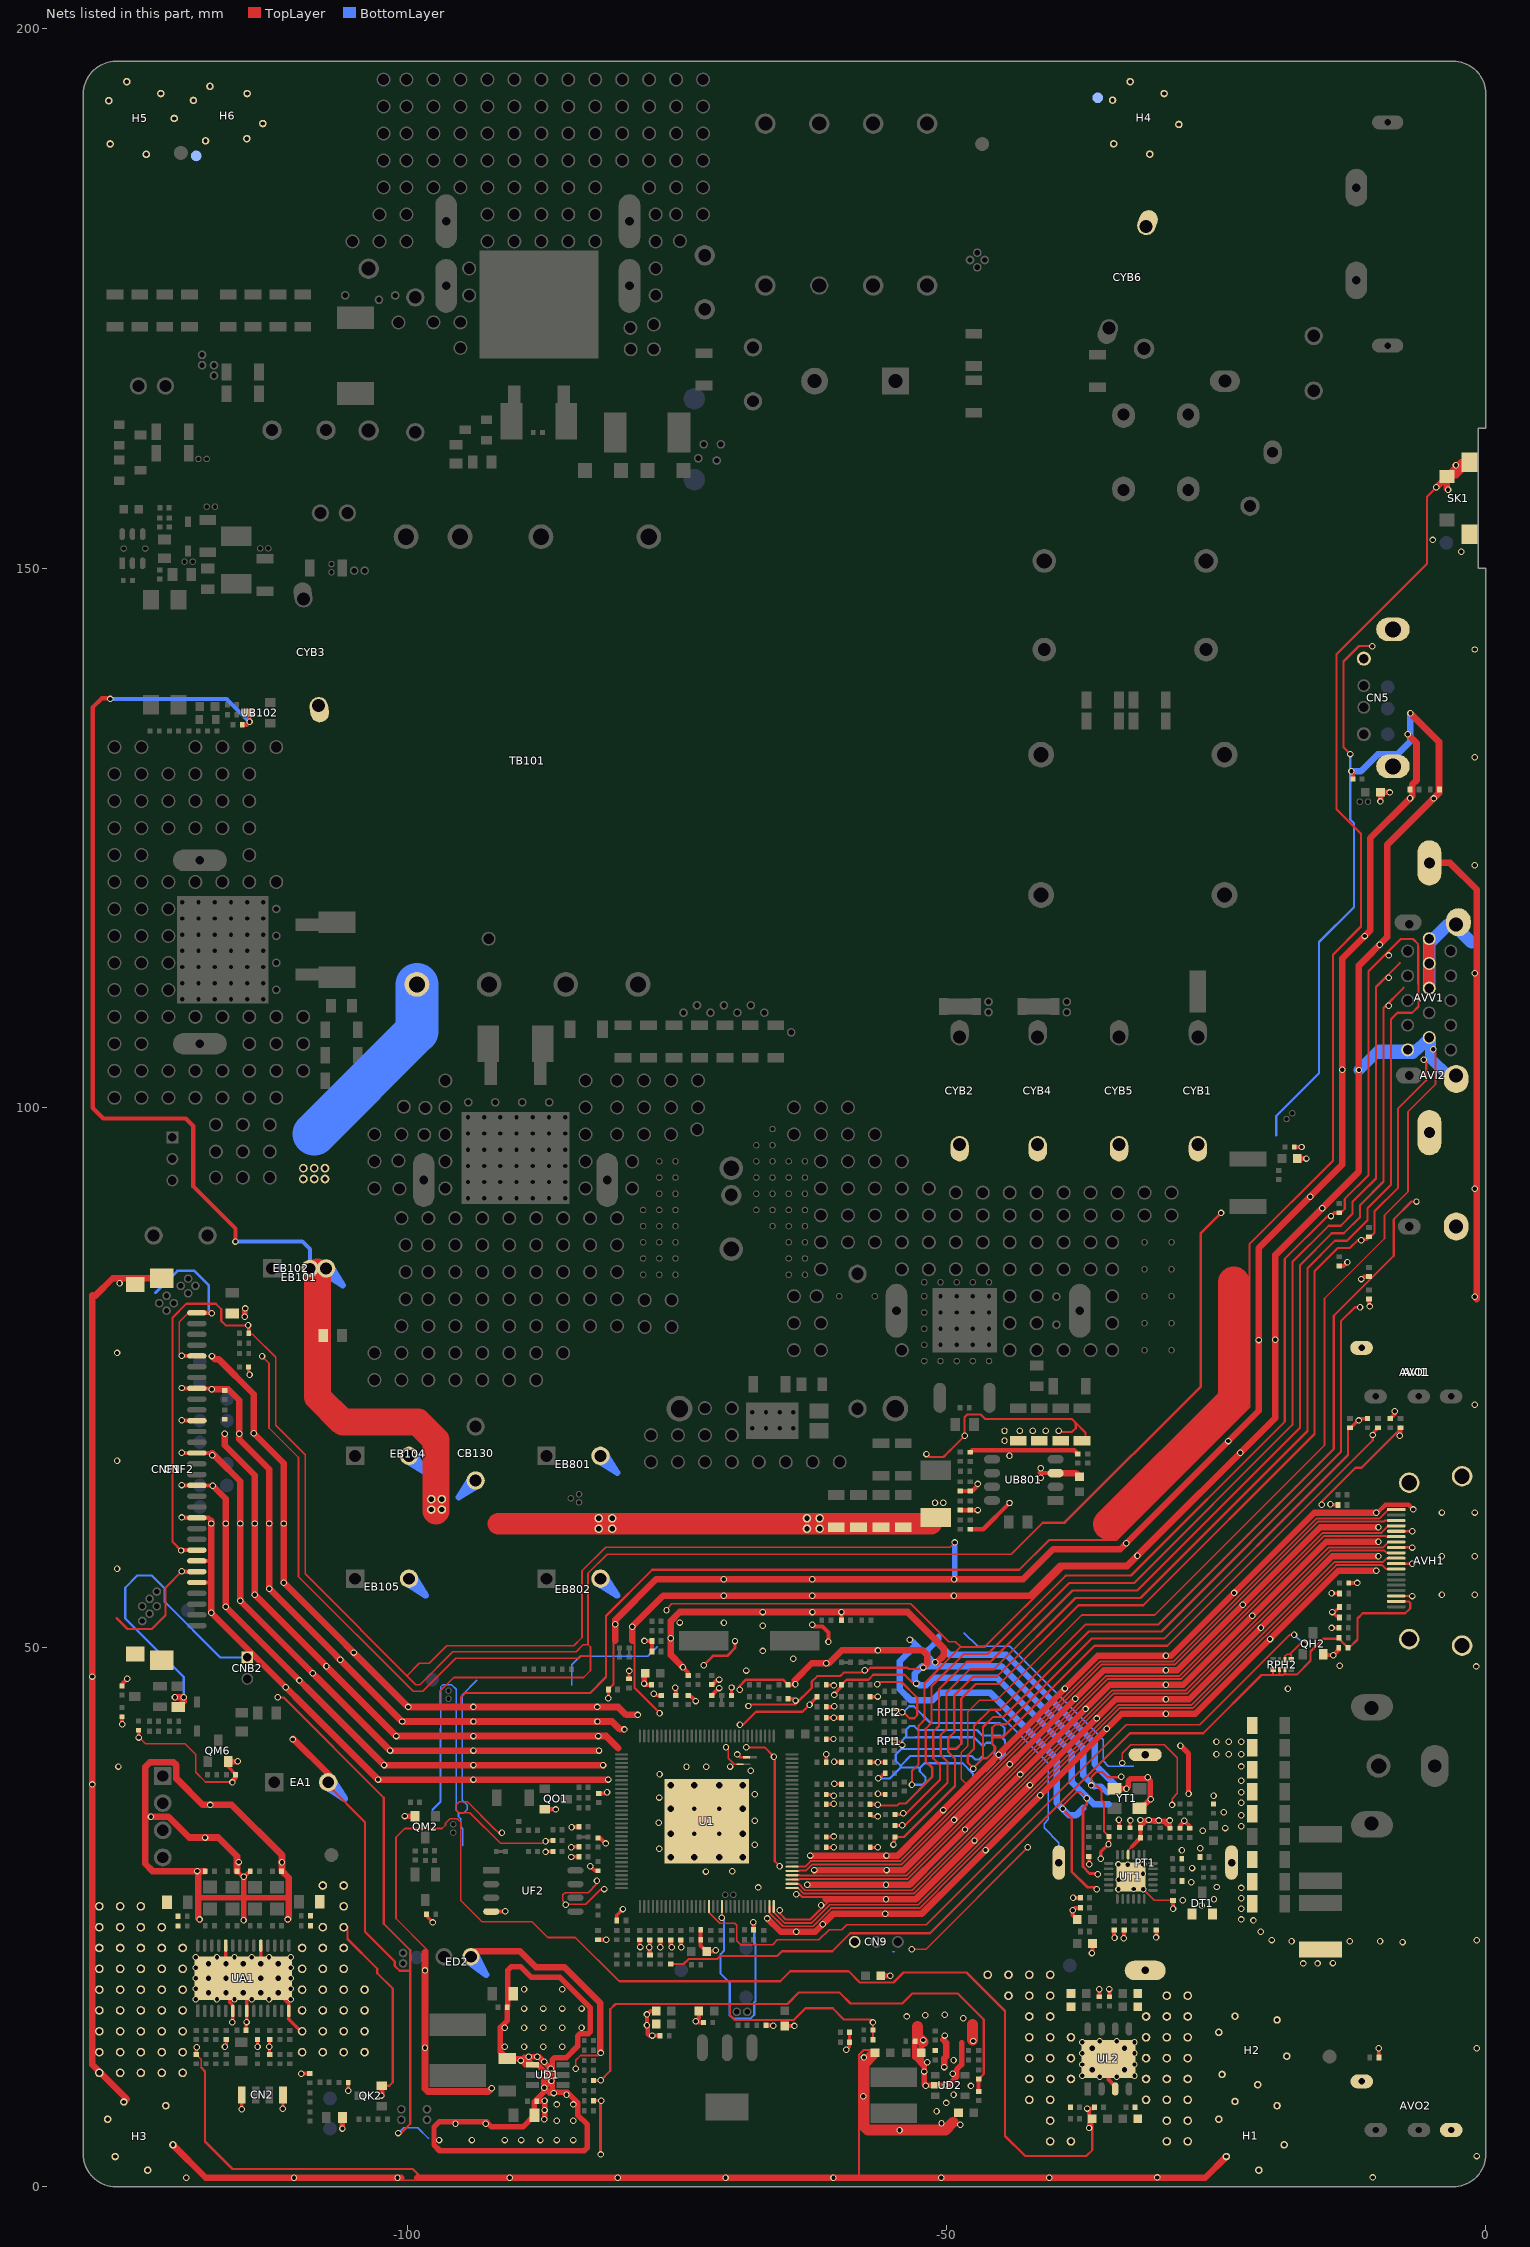
[diagram p0: the nets of this part, all layers, seen from the top]
# Altium PCB MISC84438.PcbDoc (part 10 of 15)
Units mm, origin at the board's own origin, x right, y up, seen from the top; angles counter-clockwise.
Board outline 130 x 197 mm, 2 copper layers (TopLayer, BottomLayer), stack 1.571 mm thick; 574 components, 314 nets, 2636 pads, 811 vias.

## Via types
v1: diameter 0.6, hole 0.4, TopLayer to BottomLayer, tented both sides, 780 vias
v2: diameter 0.7, hole 0.5, TopLayer to BottomLayer, tented both sides, 15 vias
v3: diameter 0.8, hole 0.6, TopLayer to BottomLayer, tented both sides, 12 vias
v4: diameter 0.8, hole 0.5, TopLayer to BottomLayer, tented both sides, 4 vias

## Nets (pads, with @x,y where several pads share a name; then routed paths per layer and width w, separated by ;. In a path a pad name is that pad's centre, name@x,y a point inside that pad or via, vN(x,y) a via of type N, cw(c..) or ccw(c..) an arc to the next point about the centre after c; other vN are vias at no path point) (continued)
GND: (continued)
  TopLayer w0.381: CF38.2@-126.416,43.555 -126.416,42.901 v1(-126.39,42.875) ; CM4.2@-126.416,46.412 -126.416,46.584 v1(-125.933,47.066) ; v1@-120.913,59 CNF2.23@-119.486,59 ; v1(-120.886,57.029) -120.857,57 CNF2.25@-119.486,57 ; v1(-120.886,62.029) -120.857,62 CNF2.20@-119.486,62 -118.413,62 v1@-118.154,61.741 ; v1(-120.886,65.029) -120.857,65 CNF2.17@-119.486,65 -118.04,65 v1(-118.001,64.96) ; v1(-120.886,68.029) -120.857,68 CNF2.14@-119.486,68 -118.31,68 -118.102,67.793 v1(-118.051,67.793) ; v1(-120.886,71.029) -120.857,71 CNF2.11@-119.486,71 ; v1(-120.886,74.029) -120.857,74 CNF2.8@-119.486,74 -118.196,74 v1(-118.11,73.914) ; v1(-120.886,77.029) -120.857,77 CNF2.5@-119.486,77 ; CNF2.26@-119.486,56 -118.115,56 ; CNF2.24@-119.486,58 -118.115,58 ; CNF2.1@-119.486,81 -118.115,81 v1@-118.086,80.971 ; v1(-116.18,37.465) -116.18,37.554 -115.882,37.852 ; CA5.2@-115.766,29.248 -115.245,28.727 v1(-115.138,28.727) -115.054,28.727 CA10.2@-114.533,29.248 ; v1(-109.791,10.477) -109.786,10.483 CK4.2@-109.004,10.483 ; UF2.4@-92.19,25.502 -90.932,25.502 v1(-90.907,25.527) ; -89.035,11.301 UD1.1@-88.356,11.301 ; QO1.E@-87.224,34.986 -86.243,34.986 v1(-86.22,34.963) ; v1(-84.747,33.325) -84.722,33.35 R1.2@-84.067,33.35 ; DH9.A@-82.296,22.889 -81.53,22.889 v1(-81.521,22.898) ; R2.2@-82.296,32.327 -82.112,32.327 v1@-81.594,31.809 ; CF6.1@-82.22,36.442 -81.566,36.442 v1(-81.458,36.551) ; CF18.1@-78.435,22.889 -78.435,22.273 v1(-78.372,22.21) ; v1(-78.029,46.634) -77.902,46.507 CF16.1@-77.336,46.507 ; v1(-77.991,50.584) -77.975,50.569 DT2.A@-77.304,50.569 DT3.A@-77.304,49.603 ; DK1.A@-77.495,21.479 -77.495,22.159 v1(-77.534,22.197) -77.483,22.248 CK2.2@-77.483,22.877 ; CL4.1@-76.91,16.281 -77.445,16.281 v1(-77.762,15.964) v1(-77.762,14.948) -77.686,14.872 -77.686,14.122 -77.572,14.008 v1(-77.267,14.008) -77.261,14.002 CL3.1@-76.542,14.002 ; v1(-76.517,22.197) RH29.2@-76.517,22.877 ; CF21.1@-75.552,22.877 -75.552,22.298 v1(-75.451,22.197) ; v1@-75.133,46.228 -75.082,46.177 CF23.1@-75.082,45.535 ; CF7.1@-74.613,22.877 -74.613,22.222 v1(-74.587,22.197) ; v1@-74.547,48.281 v1(-74.422,48.156) -73.939,47.673 CF1.1@-73.939,47.368 ; CF19.1@-73.939,45.535 -73.755,45.535 v1(-73.228,45.009) ; CL1.1@-72.944,16.281 -72.944,15.626 v1(-73.228,15.342) -73.101,15.215 CL2.1@-72.51,15.215 ; CF24.1@-72.778,23.81 CF25.1@-72.778,22.872 -72.778,22.339 CF22.2@-72.23,21.79 -71.501,21.79 v1(-71.374,21.917) ; CF12.1@-71.755,45.535 -71.755,45.545 -71.084,46.215 v1(-71.044,46.215) ; CF4.1@-71.755,46.539 CF4.1@-71.681,46.539 ; CF4.1@-71.512,46.709 CF4.1@-71.681,46.539 ; v1(-71.044,47.003) -71.218,47.003 CF4.1@-71.681,46.539 ; v1(-67.894,24.521) -67.876,24.502 CF17.1@-67.876,23.81 ; RL2.2@-66.733,14.961 -66.103,14.961 v1(-66.053,14.91) ; CF37.2@-64.973,14.889 -64.092,14.889 v1(-64.084,14.897) ; v1(-62.446,52.095) -62.272,51.922 -61.497,51.922 -60.935,51.359 v1(-60.935,50.495) ; CO5.1@-61.145,44.475 v1@-60.453,44.475 ; v1(-60.452,43.459) RO4.1@-59.734,43.459 ; CF39.1@-59.734,52.489 -59.734,53.258 v1(-59.728,53.264) ; CD12.2@-47.015,8.82 RD7.1@-47.015,9.964 ; v1@-38.265,26.772 CT18.1@-37.585,26.772 ; CT6.2@-37.867,24.765 -38.303,25.202 v1(-38.303,25.629) -38.087,25.845 CT5.1@-37.585,25.845 ; v1(-36.779,5.436) -36.779,7.061 v1(-36.957,7.239) -36.404,7.239 CL6.1@-36.277,7.366 ; v1(-36.512,21.653) -36.454,21.712 CT3.2@-36.454,22.543 ; v1(-35.839,18.288) -35.827,18.275 CL10.1@-35.827,17.595 ; UL2.EPAD@-34.989,11.836 -34.989,9.936 -34.353,9.301 UL2.3@-34.353,9.054 ; v1(-34.9,18.313) -34.887,18.301 CL13.2@-34.887,17.595 ; CT12.2@-34.461,23.781 -34.461,23.12 v1(-34.417,23.076) ; v1(-33.553,23.038) -33.533,23.058 CT11.1@-33.533,23.781 ; -32.798,31.54 -31.997,32.341 CT26.1@-31.997,32.346 CT29.1@-31.997,33.274 ; v1(-30.569,23.101) -30.544,23.127 CT9.2@-30.544,23.781 ; v1@-28.981,25.87 LT6.2@-28.981,26.537 ; CT7.1@-28.346,33.216 -28.346,33.452 -27.965,33.833 v1(-27.965,33.909) -27.432,33.376 CT8.1@-27.432,33.216 ; CU3.2@-17.761,96.368 v1(-17.079,96.368) ; QH2.E@-15.075,49.352 -14.986,49.263 v1(-14.135,49.263) -13.633,49.765 CH9.1@-13.633,49.962 ; DV1.A@-13.589,85.351 -13.176,85.351 v1(-12.827,85.7) ; CH10.1@-12.707,55.956 v1@-11.913,55.956 ; v1(-12.459,131.191) -12.312,131.045 CU2.2@-12.312,130.48 ; v1(-11.557,84.125) -11.532,84.125 -11.296,84.36 DV2.A@-10.82,84.36 ; DI1.A@-10.82,82.277 -10.82,81.636 v1(-10.77,81.585) ; v1(-10.16,62.471) -10.043,62.471 -9.307,63.208 -7.149,63.208 v1(-6.714,62.772) ; CI11.2@-8.865,71.189 -8.433,71.621 v1(-8.433,71.882) ; v1(-7.976,69.596) -7.899,69.672 DO3.A@-7.899,70.339 ; CT29.1@-31.997,33.274 CT29.1@-31.997,33.348 ; CT29.1@-31.997,33.274 -31.997,33.966 v1(-32.017,33.985) v1(-31.242,33.985) ; CT29.1@-31.997,33.348 -31.504,33.841 -30.791,33.841 -30.759,33.81 -29.806,33.81 -29.273,33.277 CT25.2@-29.273,33.216 -29.273,33.922 v1(-29.299,33.947) v1(-30.328,33.947) -30.366,33.985 v1(-31.242,33.985) ; CT29.1@-31.997,33.348 -31.36,33.985 v1(-31.242,33.985)
  TopLayer w0.4: v1@-127.5,137.954 -128.302,137.954 -129.14,137.116 -129.14,100.006 -128.149,99.016 -120.516,99.016 -119.8,98.3 -119.8,92.7 -115.9,88.8 v1(-115.9,87.6) ; RB134.1@-115.275,135.5 -114.87,135.5 v1(-114.598,135.773) -114.598,136.584 UB102.A@-114.557,136.625 ; RB803.1@-48.73,62.707 CB806.2@-47.803,62.707 -47.097,62.707 v1(-47.092,62.713) ; CB805.1@-48.73,64.485 -47.608,64.485 -47.092,65.001 v1(-47.092,65.138) ; CB813.1@-47.803,60.941 -46.577,60.941 pad.VIA5@-44.146,63.372 ; CB804.2@-47.803,68.078 -47.631,68.25 -45.009,68.25 -38.149,68.25 CB803.2@-37.821,67.921 ; -41.377,66.142 UB801.3@-39.874,66.142
  TopLayer w0.5: v1(-115.034,80.634) -115.034,81.366 v1(-115,81.4) ; v1(-28.304,40.873) -27.559,40.128 v1(-27.559,36.424) ; CU4.1@-17.48,95.301 v1(-16.627,95.301)
  TopLayer w0.508: -119.202,26.759 -111.176,26.759 ; QM6.E@-116.573,39.395 -115.71,39.395 v1(-115.684,39.421) ; v1(-115.151,24.689) -115.139,24.7 -115.139,28.726 v1(-115.138,28.727) ; v1(-105.981,5.385) -105.98,5.386 DK20.K@-105.98,6.417 ; v1(-102.375,8.445) -102.349,8.471 QK2.E@-102.349,9.36 ; v1(-100.203,34.353) -100.185,34.335 QM2.E@-99.263,34.335 ; CD41.1@-90.856,11.836 -88.89,11.836 UD1.1@-88.356,11.301 -87.892,11.301 -87.338,10.748 -87.338,8.726 -88.188,7.876 CD1.2@-88.188,6.629 -89.267,5.55 -92.163,5.55 -92.62,6.007 -97.029,6.007 -97.498,5.538 -97.498,3.861 -96.965,3.327 -83.579,3.327 -83.279,3.627 -83.279,5.743 -84.177,6.641 -84.177,7.786 -85.136,8.745 -86.313,8.745 -86.537,8.969 -86.537,11.734 -86.313,11.957 -85.232,11.957 -84.177,13.013 -84.177,13.959 -83.953,14.182 -83.198,14.182 -83.029,14.351 -83.029,16.598 -85.821,19.39 -88.463,19.39 -89.47,20.397 -90.323,20.397 -90.678,20.042 -90.678,16.76 -90.7,16.737 -90.7,16.599 -90.687,16.586 -90.687,15.422 -91.351,14.759 -91.351,12.512 CD41.1@-90.716,11.877 ; -89.035,11.301 -89.417,11.684 v1(-89.459,11.684) -89.129,12.014 -88.748,12.014 v1(-88.722,12.04) v1(-87.922,12.04) -87.757,12.04 v1(-87.287,11.57) -86.677,10.96 v1(-86.677,10.947) v1(-87.274,10.351) -86.716,9.792 v1(-86.614,9.792) -87.236,9.169 v1(-87.287,9.169) -86.792,8.674 v1(-86.411,8.674) ; CD19.2@-87.967,7.925 -87.274,7.925 v1(-87.249,7.95) v1(-87.249,7.099) -87.249,6.274 v1(-87.274,6.248) ; v1(-78.029,46.634) -78.029,47.468 CF15.2@-77.922,47.574 ; CF5.2@-56.088,19.558 v1(-55.194,19.558) ; CD16.1@-52.89,13.513 CD16.1@-52.915,13.487 ; -48.586,13.318 -48.586,11.32 -49.061,10.845 -49.061,10.172 -49.848,9.385 UD2.2@-51.03,9.385 -51.905,9.385 v1(-51.93,9.36) -52.057,9.487 -52.057,11.138 ; YT1.4@-34.415,36.879 -33.326,36.879 v1(-33.312,36.893) -33.146,37.059 -33.146,37.587 -32.923,37.81 -31.307,37.81 -31.084,37.587 -31.084,35.936 v1(-31.064,35.916) -31.901,35.079 YT1.2@-32.115,35.079 ; v1(-9.766,128.397) -9.758,128.405 CU1.1@-9.758,129.261 -8.928,129.261 v1(-8.903,129.235) ; CD16.1@-52.915,13.487 -52.248,13.487 -52.184,13.424 -52.321,13.287 -52.321,11.402 -52.057,11.138 ; CD16.1@-52.915,13.487 -52.915,11.996 -52.057,11.138
  TopLayer w0.6: v1@-110.541,41.504 -107.304,38.267 EA1.2@-107.304,37.486 ; ED2.2@-94.076,21.311 -93.576,21.811 -89.525,21.811 -88.065,20.35 -85.423,20.35 -82.069,16.996 -82.069,12.422 v1(-82.042,12.395) ; UB801.3@-39.874,66.142 -37.991,66.142 CB801.1@-37.668,65.819
  TopLayer w0.61: -129.175,82.601 -129.175,11.32 -125.97,8.115 ; -128.875,82.601 -127.275,84.2 CNF2.32@-122.736,84.2 ; v1@-124.028,34.287 -122.115,34.287 -120.188,32.36 -117.492,32.36 -115.756,30.624 CA5.2@-115.756,29.248 ; H3.5@-121.696,3.872 -118.65,0.826 -100.559,0.826 ; v1(-121.514,45.364) v1(-120.701,45.364) -120.701,44.957 CM5.1@-121.196,44.462 ; v1@-119.356,29.253 -119.356,24.893 v1(-119.228,24.765) ; CA4.2@-118.779,29.248 -118.783,29.253 -123.601,29.253 -124.269,29.921 -124.269,38.9 -123.842,39.327 -121.632,39.327 -121.379,39.074 -121.379,37.825 -118.936,35.382 -116.24,35.382 -111.591,30.733 -111.591,29.248 -110.969,28.627 -110.969,24.845 v1(-111.049,24.765) ; v1@-118.154,61.741 v1(-118.154,53.201) v1(-102.684,37.731) v1(-81.342,37.731) ; v1@-118.153,73.906 -116.565,73.906 -115.549,72.89 -115.549,69.279 -112.769,66.499 v1(-112.769,55.432) v1(-100.454,43.116) -80.989,43.116 -80.252,42.38 v1(-79.844,42.38) ; v1(-118.084,76.987) -117.78,76.683 -117.438,76.683 -114.203,73.448 v1(-114.203,69.836) -111.423,67.056 v1(-111.423,55.989) v1(-99.896,44.462) -80.431,44.462 -79.695,43.726 v1(-78.623,43.726) ; v1@-118.078,68 -117.516,67.438 -115.462,65.383 v1(-115.462,54.317) v1(-101.569,40.424) v1(-82.202,40.424) ; v1(-118.001,64.96) -116.808,63.768 v1(-116.808,53.759) v1(-102.126,39.078) v1(-81.826,39.078) ; v1(-116.896,69.799) -116.896,68.721 -114.115,65.941 v1(-114.115,54.874) v1(-101.011,41.77) -81.546,41.77 -80.429,40.653 ; -99.047,0.826 -26.011,0.826 H1.1@-24.05,2.786 ; -98.333,21.73 -98.333,9.07 -98.08,8.817 -92.452,8.817 v1(-92.138,9.131) ; -80.683,50.597 -80.683,52.534 -76.905,56.312 -42.882,56.312 -40.113,59.08 -33.89,59.08 -21.057,71.914 -21.057,87.002 -13.31,94.749 -13.31,113.841 -10.706,116.444 -10.706,125.002 v1(-7.022,128.685) -6.836,128.872 -6.836,129.942 -6.426,130.351 -6.426,133.812 v1(-7.237,134.622) ; -79.134,50.622 v1(-79.134,51.892) -76.263,54.762 -42.24,54.762 -39.472,57.531 -33.249,57.531 -19.507,71.272 -19.507,86.36 -11.76,94.107 -11.76,113.199 -9.157,115.802 -9.157,124.36 -4.343,129.173 -4.343,133.92 v1(-6.986,136.563) ; v1@-74.547,48.281 -75.543,49.277 -75.543,52.435 -74.714,53.264 -53.594,53.264 -50.267,49.936 -50.267,49.2 -50.863,48.603 v1(-51.029,48.603) ; v1(-66.605,24.86) -65.363,23.619 -62.151,23.619 -60.465,25.305 -52.268,25.305 -48.629,28.944 -33.745,43.828 -26.93,43.828 -13.671,57.087 v1(-10.154,57.087) ; v1@-64.047,46.562 -64.047,46.941 -62.474,48.514 -60.896,48.514 -59.707,49.703 -52.199,49.703 -51.77,49.274 -51.77,48.488 v1(-52.142,48.116) ; v1(-62.896,27.998) -53.383,27.998 -50.533,30.848 -34.86,46.52 -28.045,46.52 -14.786,59.779 v1(-9.957,59.779) ; v1(-62.63,30.69) -54.498,30.69 -52.437,32.752 -35.976,49.212 -29.16,49.212 -15.901,62.471 v1(-10.16,62.471) ; v1(-62.238,29.344) -53.941,29.344 -51.485,31.8 -35.418,47.866 -28.602,47.866 -15.344,61.125 v1(-9.957,61.125) ; -61.177,26.651 -52.825,26.651 -49.581,29.896 -34.303,45.174 -27.487,45.174 -14.228,58.433 v1(-9.957,58.433) ; -50.297,13.607 -50.015,13.325 -50.015,12.064 -50.203,11.875 v1(-50.203,11.087) ; AVV1.17@-5.227,122.7 -3.32,122.7 -0.826,120.206 v1@-0.826,82.271 ; v1@-4.585,157.518 SK1.1@-3.603,158.5 ; v1(-3.505,157.302) -3.603,157.4 SK1.1@-3.603,158.5 ; v1(-2.773,159.552) -2.773,159.381 -3.603,158.551 SK1.1@-3.603,158.5 ; SK1.4@-2.253,159.85 SK1.1@-3.603,158.5 ; SK1.4@-1.528,159.85 -2.745,158.634 -3.469,158.634 SK1.1@-3.603,158.5
  TopLayer w1.016: CD15.1@-56.8,12.233 -57.649,11.383 -57.649,5.632 -57.277,5.261 -50.081,5.261 -49.373,5.969 ; -52.667,14.831 -52.667,13.906 v1@-52.184,13.424 ; v1@-47.604,13.602 -47.604,15.044 ; AVV1.8@-5.247,111.095 AVV1.6@-5.247,115.675
  TopLayer w2: -91.553,61.454 DB804.K@-51.41,61.454
  TopLayer w2.5: EB102.2@-108.3,84.8 -108.3,73.207 -105.948,70.856 -98.986,70.856 -97.333,69.202 -97.333,62.636
  TopLayer w2.95: -34.93,61.394 -23.37,72.954 -23.37,83.83
  BottomLayer w0.127: -51.258,44.209 -45.514,44.209 -40.547,39.242 -40.547,34.035 -40.927,33.655 -40.927,33.249 -39.572,31.894 PT1.4@-39.572,30.041 ; -48.389,51.361 -47.104,50.076 -44.138,50.076 -35.48,41.418 -35.48,39.462 -34.976,38.959 -32.654,38.959
  BottomLayer w0.152: v1(-100.813,4.966) -100.309,5.469 -99.004,5.469 -98.006,4.47 ; -96.888,42.456 -96.888,46.317 -96.698,46.507 -95.857,46.507 -95.441,46.091 -95.441,34.874 -95.225,34.658 ; -94.831,31.585 -94.831,33.185 -95.009,33.363 -95.009,34.099 -95.225,34.315 -95.225,34.663 -94.724,34.663 -94.429,34.958 -94.429,35.375 -94.882,35.827 -94.882,45.58 -93.523,46.939 ; -84.734,46.482 -84.734,48.362 -83.929,49.167 -77.681,49.167 -76.81,50.038 ; -54.991,21.76 -54.831,21.76
  BottomLayer w0.203: v1(-120.701,45.364) -120.701,47.244 -126.124,52.667 -126.124,55.524 -124.993,56.655 -123.661,56.655 -122.453,55.447 -122.453,54.203 -117.307,49.057 CNB2.1@-114.808,49.057 ; -97.638,34.925 -96.888,35.674 -96.888,42.456 ; v1(-70.815,24.915) -70.613,24.712 -70.613,21.857 -70.929,21.54 -70.929,19.743 -70.079,18.892 -70.079,15.895 -69.741,15.557 -68.193,15.557 -67.815,15.936 -67.815,17.083 -67.704,17.194 -67.704,22.481 -67.815,22.592 -67.815,24.441 v1(-67.894,24.521) ; v1(-56.81,15.22) v1@-56.794,15.204 ; v1(-56.325,37.841) -55.235,37.841 -54.232,38.844 ; v1(-54.102,40.932) -54.102,41.364 -53.837,41.629 ; v1(-54.102,43.967) -54.011,43.967 -53.457,44.521 -53.019,44.521 -51.483,42.985 -45.08,42.985 -44.628,42.532 -44.628,41.923 -44.882,41.669 ; v1(-53.196,37.247) -52.224,37.247 -51.943,37.529 -51.943,37.959 -52.476,38.492 -52.476,38.824 ; -48.882,41.664 -48.616,41.397 -48.616,41.061 -49.105,40.572 -54.181,40.572 -54.699,40.054 -54.699,39.489 -54.232,39.022 ; -48.336,36.678 -47.549,37.465 -47.549,38.303 -48.496,39.251 -52.029,39.251 -52.435,38.844 -54.232,38.844 ; -46.304,38.583 -45.547,39.34 -45.547,40.834 -45.857,41.143 -46.295,41.143 -46.607,40.831 -46.607,40.824 ; -45.021,39.649 -44.569,40.102 -44.569,41.354 -45.018,41.804 -46.653,41.804 -47.174,42.324 -52.616,42.324 -52.977,42.686 -53.415,42.686 -53.725,42.376 -53.725,41.741 -53.837,41.629 ; -19.421,97.429 -19.421,99.239 -15.456,103.204 -15.456,115.365 -12.217,118.604 -12.217,126.378 -12.22,126.378 -12.573,126.731 v1(-12.573,132.791) ; -54.232,38.844 -54.232,39.022 ; -54.232,39.022 -53.343,39.911 -47.653,39.911 -47.328,39.586 -46.943,39.586 -46.607,39.922 -46.607,40.824 ; -53.837,41.629 -52.872,41.629 -52.837,41.664 -47.447,41.664 -46.607,40.824
  BottomLayer w0.254: -123.311,82.861 -121.285,84.887 -119.71,84.887 -118.386,83.562 v1@-118.386,80.953
  BottomLayer w0.305: v1(-59.294,12.695) v1@-59.111,12.878
  BottomLayer w0.381: v1@-17.14,96.368 v1(-17.079,96.368)
  BottomLayer w0.4: v1(-127.5,137.897) -116.722,137.897 v1(-114.598,135.773) v1@-114.625,135.8 ; v1(-115.9,87.6) -109.7,87.6 -109,86.9 EB102.2@-109,85.114
  BottomLayer w0.5: v1@-115,81.3 v1(-115,81.4) ; v1@-16.632,95.296 v1(-16.627,95.301)
  BottomLayer w0.508: v1(-53.391,50.686) -53.253,50.686 -51.821,49.253 -51.821,48.62 -51.765,48.565 -51.727,48.603 v1(-51.029,48.603) -51.141,48.603 -51.719,49.181 -51.719,49.745 -50.711,50.753 -50.711,51.041 ; v1(-49.289,56.312) -49.233,56.367 v1(-49.233,59.71) ; v1@-36.296,37.113 -35.678,37.113 -35.052,36.487
  BottomLayer w0.61: -52.864,50.165 -54.326,48.703 -54.326,46.107 -53.291,45.072 -51.314,45.072 -50.615,45.771 -45.921,45.771 -39.785,39.635 -39.785,35.588 -38.606,34.409 -38,34.409 -37.313,35.097 ; -50.692,50.273 -49.72,49.301 -44.459,49.301 -36.255,41.097 -36.255,39.141 -34.46,37.346 ; v1@-36.296,37.113 -37.321,38.138 -37.321,40.656 -44.901,48.235 -52.254,48.235 -52.929,47.56 -52.929,46.896 -52.502,46.469 -51.892,46.469 -51.194,47.168 -45.342,47.168 -38.388,40.214 -38.388,37.509 -36.338,35.458 -34.938,35.458 ; v1(-12.459,131.191) -11.582,131.191 -9.995,132.779 -8.191,132.779 -6.986,133.984 v1(-6.986,136.563)
  BottomLayer w1.016: AVI2.4@-2.75,103 -3.522,103 -5.117,104.595 -5.117,106.385 AVV1.10@-5.247,106.515 ; AVV1.10@-5.247,106.515 -6.742,105.02 -10.245,105.02 v1(-11.76,103.505) -9.895,105.37 -6.392,105.37 AVV1.10@-5.247,106.515
  BottomLayer w1.143: AVV1.8@-5.247,111.095 -5.232,111.11 -5.232,115.279 -3.512,117 AVI2.6@-2.75,117 ; AVI2.6@-2.75,116.767 -1.314,115.331
  BottomLayer w4: -108.6,97.572 -99.085,107.087 TB101.6@-99.085,111.443
  other v1: -120.475,0.826 -110.475,0.826 -100.881,0.826 -90.475,0.826 -80.475,0.826 -70.475,0.826 -60.475,0.826 -50.475,0.826 -40.475,0.826 -30.47,0.851 -10.47,0.851 -0.838,2.835 -97.028,4.318 -93.98,4.318 -90.932,4.318 -89.408,4.318 -87.63,4.318 -86.106,4.318 -84.582,4.318 -54.343,5.22 -48.717,5.74 -95.504,5.842 -92.71,5.842 -50.457,5.88 -86.106,6.096 -84.582,6.096 -50.914,6.998 -86.106,7.62 -84.582,7.62 -50.025,7.76 -57.696,8.369 -85.217,8.509 -49.34,8.522 -47.727,9.335 -50.127,9.385 -35.779,10.183 -34.198,10.183 -37.411,10.289 -32.566,10.289 -49.416,10.452 -52.057,10.668 -37.411,11.321 -32.566,11.321 -51.791,11.519 -49.34,11.722 -57.643,11.974 -37.411,12.352 -32.566,12.352 -0.838,12.835 -98.333,12.878 -90.932,12.954 -89.154,12.954 -87.376,12.954 -85.598,12.954 -37.411,13.384 -32.566,13.384 -47.511,13.5 -35.779,13.489 -34.198,13.489 -52.133,13.589 -50.165,14.008 -90.932,14.732 -89.154,14.732 -87.376,14.732 -85.598,14.732 -83.82,14.732 -48.428,15.596 -53.67,15.778 -51.968,15.88 -50.16,15.946 -89.154,16.51 -87.376,16.51 -85.598,16.51 -83.82,16.51 -119.568,17.361 -117.617,17.367 -115.991,17.367 -114.391,17.367 -112.791,17.367 -110.782,17.361 -89.154,18.288 -85.598,18.288 -119.568,18.338 -110.782,18.338 -119.568,19.315 -110.782,19.315 -98.333,20.041 -119.568,20.291 -110.782,20.291 -16.929,20.688 -15.596,20.688 -14.173,20.726 -119.568,21.268 -117.617,21.274 -115.991,21.274 -114.391,21.274 -112.791,21.274 -110.782,21.268 -7.722,22.669 -18.009,22.733 -12.624,22.733 -9.804,22.733 -0.838,22.835 -19.837,22.86 -63.919,23.619 -20.866,23.635 -61.452,24.317 -21.539,24.676 -22.682,24.765 -55.664,25.305 -28.994,25.756 -22.682,25.756 -61.62,26.071 -26.352,26.06 -28.105,26.543 -25.197,26.632 -55.601,26.651 -22.682,26.733 -38.265,26.772 -34.055,27.564 -31.756,27.564 -32.626,27.589 -22.682,27.686 -67.45,27.737 -24.93,27.775 -55.601,27.998 -27.318,28.219 -34.03,28.434 -31.781,28.994 -72.288,29.21 -119.431,29.253 -69.863,29.248 -55.55,29.344 -27.229,29.527 -33.186,29.839 -34.055,29.864 -31.756,29.864 -115.595,30.086 -111.591,30.074 -55.562,30.69 -46.373,31.2 -28.169,31.191 -76.619,31.331 -26.467,31.369 -60.452,31.445 -67.767,31.699 -81.568,31.809 -47.397,32.079 -118.72,32.36 -73.362,32.721 -71.062,32.721 -26.251,32.995 -48.276,33.104 -24.143,33.236 -22.682,33.401 -76.67,33.718 -67.78,33.922 -49.291,33.993 -123.736,34.287 -22.682,34.43 -24.282,34.709 -50.284,34.904 -73.362,35.021 -71.062,35.021 -118.237,35.382 -56.371,35.391 -60.452,35.484 -22.682,35.573 -76.619,36.068 -25.235,36.22 -41.292,36.281 -67.767,36.373 -56.347,36.414 -22.682,36.551 -42.254,37.222 -129.175,37.28 -22.682,37.63 -93.84,37.731 -31.344,37.948 -76.594,38.214 -43.169,38.211 -68.123,38.557 -74.092,38.913 -72.263,38.913 -126.746,38.938 -70.053,38.938 -22.682,38.951 -93.84,39.078 -44.137,39.147 -45.162,40.026 -24.968,40.094 -23.825,40.094 -22.682,40.094 -93.84,40.424 -24.968,41.237 -23.825,41.237 -22.682,41.237 -110.592,41.453 -93.84,41.77 -82.283,41.77 -35.127,42.446 -93.84,43.116 -82.347,43.116 -36.079,43.398 -29.654,43.828 -37.103,44.277 -93.84,44.462 -82.359,44.462 -29.654,45.174 -38.063,45.221 -18.339,46.152 -39.015,46.173 -75.133,46.253 -111.247,46.295 -29.654,46.52 -109.968,46.919 -129.175,47.28 -108.725,47.58 -68.567,47.841 -29.654,47.866 -107.464,48.223 -0.876,48.222 -13.551,48.273 -61.138,48.514 -106.175,48.838 -64.186,48.92 -29.654,49.212 -104.942,49.509 -67.018,49.657 -56.35,49.703 -19.999,50.758 -75.543,50.838 -20.844,51.817 -67.018,51.981 -80.683,52.133 -70.625,52.261 -74.714,52.286 -21.64,52.925 -67.018,53.264 -62.42,53.264 -22.532,53.936 -70.637,54.762 -62.446,54.762 -49.301,54.762 -4.064,54.864 -1.016,54.864 -14.3,54.991 -23.341,55.032 -11.913,55.956 -70.637,56.312 -62.433,56.312 -126.875,57.28 -4.064,58.42 -1.016,58.42 -32.291,58.489 -33.321,59.65 -118.154,61.468 -116.808,61.468 -115.462,61.468 -114.115,61.468 -112.769,61.468 -111.423,61.468 -4.064,62.484 -1.016,62.484 -14.402,63.246 -126.875,67.28 -22.766,68.013 -23.862,69.109 -115.549,69.799 -11.786,71.018 -1.016,72.484 -126.875,77.28 -21.057,78.473 -19.507,78.511 -118.086,80.953 -1.016,82.484 -126.644,83.744 -15.171,90.696 -16.288,91.77 -1.016,92.484 -13.31,103.518 -8.992,109.449 -8.992,112.065 -1.016,112.484 -8.992,114.122 -9.839,115.12 -11.231,115.919 -1.016,122.484 -4.836,128.68 -1.016,132.484 -1.016,142.484 -2.286,151.536 -4.915,152.641 -4.585,157.518
  other v2: -118.401,17.965 -116.775,17.965 -115.175,17.965 -113.575,17.965 -111.949,17.965 -118.401,19.315 -116.775,19.315 -113.575,19.315 -111.949,19.315 -118.401,20.664 -116.775,20.665 -115.175,20.665 -113.575,20.665 -111.949,20.665
  other v3: -75.543,30.539 -73.362,30.539 -71.062,30.539 -68.881,30.539 -75.543,32.721 -68.881,32.721 -75.543,35.021 -68.881,35.021 -75.543,37.202 -73.362,37.202 -71.062,37.202 -68.881,37.202
  other v4: -36.488,10.836 -33.488,10.836 -36.489,12.836 -33.488,12.836
HDMI1_5V: AVH1.18 CH9.2 RH14.2 RH28.2 RPH2.1 RPH2.3 RPH2.5 | length 88
  TopLayer w0.203: RH28.2@-75.553,20.629 -74.366,20.629 -73.897,21.098 -71.234,21.098 -70.955,21.377 -65.682,21.377 -65.244,21.816 -60.578,21.816 -58.911,23.482 -51.524,23.482 -33.486,41.52 -32.982,42.024 -26.183,42.024 -20.785,47.422 -19.66,47.422 ; RPH2.1@-19.722,47.937 -19.722,47.484 -19.66,47.422 ; RPH2.3@-19.122,47.937 -19.122,47.426 -19.126,47.422 ; RPH2.5@-18.622,47.937 -18.622,47.57 ; RH14.2@-13.608,50.876 RH14.2@-13.608,50.786 ; AVH1.18@-8.3,54.25 -7.163,54.25 -7.01,54.098 -7.01,53.594 -7.463,53.141 -11.413,53.141 -11.887,52.667 -11.887,50.724 -12.649,49.962 CH9.2@-12.783,49.962 RH14.2@-13.608,50.786 ; -19.66,47.422 -19.126,47.422 ; -19.126,47.422 -18.771,47.422 -18.622,47.57 ; -18.622,47.57 -18.51,47.458 -17.534,47.458 -16.256,48.736 -16.256,49.606 -15.076,50.786 RH14.2@-13.608,50.786
HDMI1_HPDIN: RPH2.6 RPH2.8 U1.113 | length 73.1
  TopLayer w0.127: U1.113@-72.012,25.971 -72.012,25.418 -71.018,24.424 -69.601,24.424 -69.421,24.244 -69.421,22.796 -69.056,22.432 -66.119,22.432 -65.68,22.87 -61.84,22.87 -60.881,23.829 -59.696,23.829 -59.243,24.282 -51.855,24.282 -33.716,42.422 -33.313,42.824 -26.514,42.824 -25.489,43.85 -18.17,51.168 v1(-17.78,51.168) ; RPH2.6@-18.622,48.837 -18.622,49.141 -18.399,49.365 -18.11,49.365 ; RPH2.8@-18.022,48.837 -18.022,49.277 -18.11,49.365 ; v1(-16.891,50.305) -17.197,50.305 -18.11,49.391 -18.11,49.365
  BottomLayer w0.127: v1(-17.78,51.168) -17.755,51.168 v1(-16.891,50.305)
HDMI1_RX0_N: AVH1.9 U1.1 | length 69.5
  TopLayer w0.178: U1.1@-64.312,27.671 -63.736,27.671 -63.238,27.172 -53.041,27.172 -49.949,30.264 -34.518,45.695 -27.703,45.695 -14.444,58.953 -9.398,58.953 -9.195,58.75 AVH1.9@-8.3,58.75
HDMI1_RX0_P: AVH1.7 U1.2 | length 69.6
  TopLayer w0.178: U1.2@-64.312,28.071 -63.705,28.071 -63.111,27.477 -53.167,27.477 -50.165,30.48 -34.645,45.999 -27.829,45.999 -14.57,59.258 -9.53,59.258 -9.038,59.75 AVH1.7@-8.3,59.75
HDMI1_RX1_N: AVH1.6 U1.3 | length 69.2
  TopLayer w0.178: U1.3@-64.312,28.471 -63.621,28.471 -63.573,28.518 -53.599,28.518 -50.901,31.216 -35.076,47.041 -28.26,47.041 -15.002,60.3 -9.296,60.3 -9.247,60.25 AVH1.6@-8.3,60.25
HDMI1_RX1_P: AVH1.4@-8.3,61.25 U1.4 | length 69.5
  TopLayer w0.178: U1.4@-64.312,28.871 -63.621,28.871 -63.573,28.823 -53.725,28.823 -51.116,31.431 -35.202,47.346 -28.387,47.346 -15.128,60.604 -9.684,60.604 -9.038,61.25 AVH1.4@-8.3,61.25
HDMI1_RX2_N: AVH1.3 U1.5 | length 69.5
  TopLayer w0.178: U1.5@-64.312,29.271 -63.621,29.271 -63.573,29.318 -62.999,29.318 -62.453,29.864 -54.156,29.864 -51.853,32.168 -35.634,48.387 -28.818,48.387 -15.559,61.646 -9.474,61.646 -9.37,61.75 AVH1.3@-8.3,61.75
HDMI1_RX2_P: AVH1.1 U1.6 | length 69.7
  TopLayer w0.178: U1.6@-64.312,29.671 -63.078,29.671 -62.579,30.169 -54.283,30.169 -52.068,32.383 -35.76,48.692 -28.944,48.692 -15.686,61.951 -9.838,61.951 -9.038,62.75 AVH1.1@-8.3,62.75
HDMI1_RXC_N: AVH1.12 U1.127 | length 73.2
  TopLayer w0.178: U1.127@-66.412,25.971 -66.412,25.404 -65.148,24.14 -62.366,24.14 -60.68,25.826 -52.483,25.826 -48.997,29.312 -33.961,44.348 -27.145,44.348 -13.886,57.607 -9.601,57.607 -9.244,57.25 AVH1.12@-8.3,57.25
HDMI1_RXC_P: AVH1.10 U1.128 | length 72.7
  TopLayer w0.178: U1.128@-66.012,25.971 -66.012,25.435 -65.021,24.445 -62.492,24.445 -60.807,26.131 -52.61,26.131 -49.213,29.528 -34.087,44.653 -27.271,44.653 -14.013,57.912 -9.525,57.912 -9.187,58.25 AVH1.10@-8.3,58.25